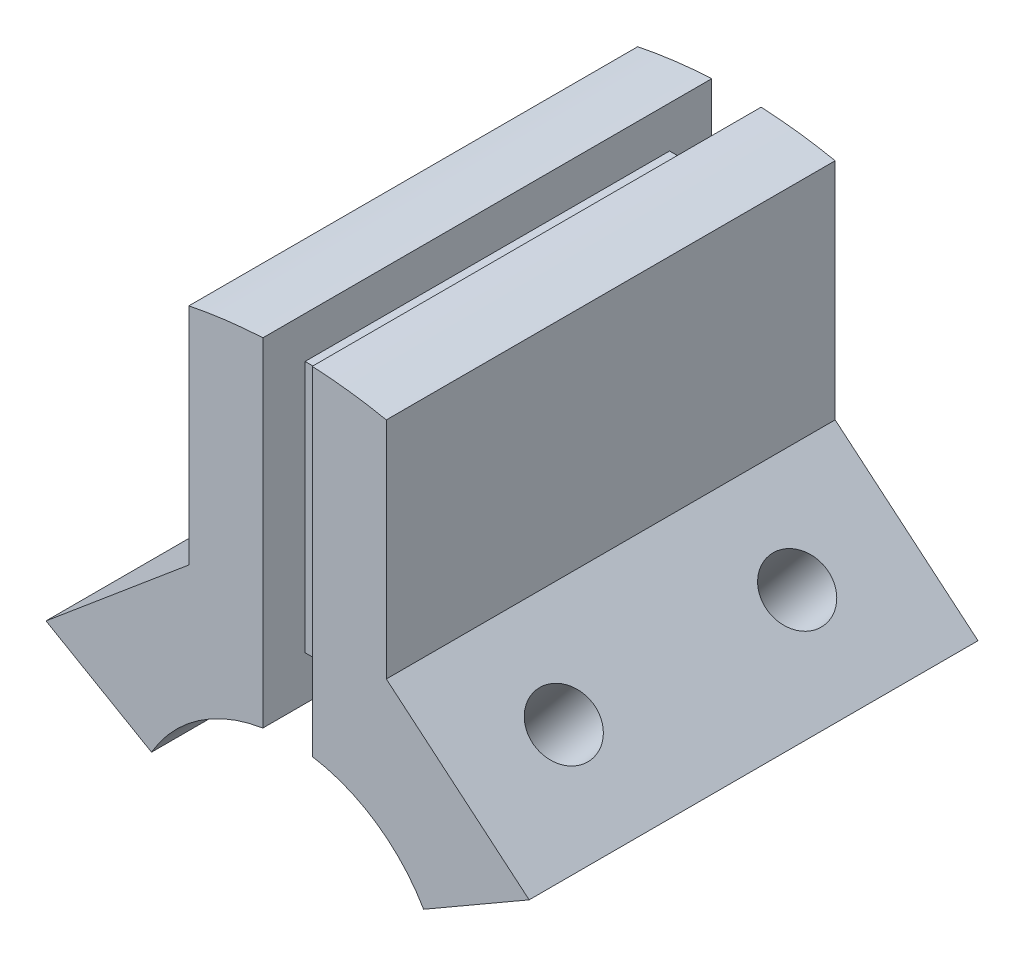
SolidWorks part; units mm, degrees
ref_plane "Front Plane" through (0, 0, 0) normal (0, 0, 1) x (1, 0, 0)
ref_plane "Top Plane" through (0, 0, 0) normal (0, 1, 0) x (1, 0, 0)
ref_plane "Right Plane" through (0, 0, 0) normal (1, 0, 0) x (0, 0, -1)
other "Configuration Table"
sketch "Sketch1" plane through (0, 0, 0) normal (0, 0, 1) x (1, 0, 0)
  line L0 (0, 0) -> (0, 85.2062) construction
  line L1 (-2.75, 54.9312) -> (-2.75, 17.2826)
  line L2 (-11, 53.8888) -> (-11, 28.8888)
  line L3 (-11, 28.8888) -> (-26.9116, 15.5374)
  line L4 (-26.9116, 15.5374) -> (-15.1554, 8.75)
  line L5 (0, 0) -> (-31.7375, 0) construction
  line L6 (11, 28.8888) -> (26.9116, 15.5374)
  line L7 (26.9116, 15.5374) -> (15.1554, 8.75)
  line L8 (2.75, 54.9312) -> (2.75, 17.2826)
  line L9 (11, 53.8888) -> (11, 28.8888)
  arc A0 (11, 53.8888) -> (2.75, 54.9312) centre (0, 0) ccw
  arc A1 (15.1554, 8.75) -> (2.75, 17.2826) centre (0, 0) ccw
  arc A2 (-2.75, 54.9312) -> (-11, 53.8888) centre (0, 0) ccw
  arc A3 (-2.75, 17.2826) -> (-15.1554, 8.75) centre (0, 0) ccw
  dimension "D1" = 110
  dimension "D2" = 35
  dimension "D3" = 2.75
  dimension "D4" = 25
  dimension "D5" = 40
  dimension "D6" = 60
  dimension "D7" = 11
extrude "Boss-Extrude1" add sketch "Sketch1" along normal mid plane 50
sketch "Sketch2" plane through (0, 0, 0) normal (0, 0, 1) x (1, 0, 0)
  line L0 (-2.75, 17.2826) -> (-2.75, 54.9312) construction
  line L1 (2.75, 22.2) -> (-2.75, 22.2)
  line L2 (2.75, 22.2) -> (2.75, 50.3)
  line L3 (2.75, 50.3) -> (-2.75, 50.3)
  line L4 (-2.75, 22.2) -> (-2.75, 50.3)
  line L5 (2.75, 22.2) -> (-2.75, 50.3) construction
  line L6 (2.75, 50.3) -> (-2.75, 22.2) construction
  point P0 (0, 36.25)
  dimension "D1" = 5.5
  dimension "D2" = 22.2
  dimension "D3" = 50.3
extrude "Boss-Extrude2" add sketch "Sketch2" along normal mid plane 40.6
ref_plane "Plane1" through (0, 0, -13) normal (0, 0, 1) x (1, 0, 0)
ref_plane "Plane2" through (0, 0, 13) normal (0, 0, 1) x (1, 0, 0)
sketch "Sketch3" plane through (0, 0, -13) normal (0, 0, 1) x (1, 0, 0)
  line L0 (0, 0) -> (0, 38.8672) construction
  line L1 (0, 0) -> (-18.7699, 22.3691) construction
  line L2 (-11, 28.8888) -> (-26.9116, 15.5374) construction
  line L3 (0, 0) -> (18.7699, 22.3691) construction
  dimension "D1" = 40
sketch "Sketch5" plane through (0, 0, 13) normal (0, 0, 1) x (1, 0, 0)
  line L0 (0, 0) -> (18.7699, 22.3691) construction
  line L1 (0, 0) -> (-18.7699, 22.3691) construction
  line L2 (0, 0) -> (18.7699, 22.3691) construction
  line L3 (0, 0) -> (-18.7699, 22.3691) construction
hole_wizard "Ø6.0mm Blind Dowel Hole1" positions "3DSketch1" profile "Sketch6" hole size "Ø6.0" standard "GB" end condition through all
sketch3d "3DSketch1"
  point P0 (-18.7699, 22.3691, -13)
  point P3 (-18.7699, 22.3691, -13)
  point P5 (-18.7699, 22.3691, -13)
  point P7 (-18.7699, 22.3691, 13)
sketch "Sketch6" plane through (-18.7699, 22.3691, 13) normal (0, 0, 1) x (-0.766, -0.6428, 0)
  line L0 (0, 0) -> (0, 39.7963)
  line L1 (0, 39.7963) -> (3, 39.7963)
  line L2 (3, 39.7963) -> (3, 0)
  line L5 (3, 0) -> (0, 0)
  line L11 (0, -6.35) -> (0, 107.95) construction
  dimension "通孔孔直径" = 6
  dimension "通孔孔深度" = 39.7963
hole_wizard "Ø6.0mm Blind Dowel Hole2" positions "3DSketch2" profile "Sketch7" hole size "Ø6.0" standard "GB" end condition through all
sketch3d "3DSketch2"
  line L0 (0, 0, 13) -> (18.7699, 22.3691, 13) construction
  point P0 (18.7699, 22.3691, 13)
  point P2 (18.7699, 22.3691, -13)
sketch "Sketch7" plane through (18.7699, 22.3691, 13) normal (0, 0, 1) x (-0.766, 0.6428, 0)
  line L0 (0, 0) -> (0, 39.7963)
  line L1 (0, 39.7963) -> (3.5, 39.7963)
  line L2 (3.5, 39.7963) -> (3.5, 0)
  line L5 (3.5, 0) -> (0, 0)
  line L11 (0, -6.35) -> (0, 107.95) construction
  dimension "通孔孔直径" = 7
  dimension "通孔孔深度" = 39.7963
